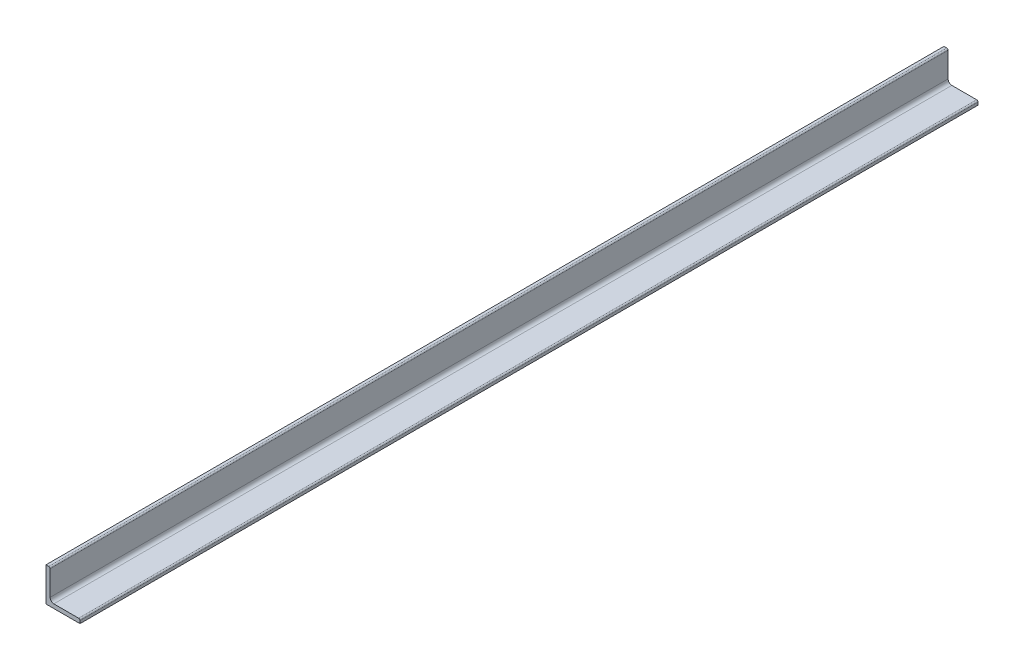
SolidWorks part; units mm, degrees
material "普通碳钢"
ref_plane "Front Plane" through (0, 0, 0) normal (0, 0, 1) x (1, 0, 0)
ref_plane "Top Plane" through (0, 0, 0) normal (0, 1, 0) x (1, 0, 0)
ref_plane "Right Plane" through (0, 0, 0) normal (1, 0, 0) x (0, 0, -1)
sketch "Sketch1" plane through (0, 0, 0) normal (0, 0, 1) x (1, 0, 0)
  line L0 (0, 50) -> (0, 0)
  line L1 (0, 0) -> (50, 0)
  line L2 (50, 0) -> (50, 4)
  line L3 (48, 6) -> (11.5, 6)
  line L4 (6, 11.5) -> (6, 48)
  line L5 (4, 50) -> (0, 50)
  arc A0 (11.5, 6) -> (6, 11.5) centre (11.5, 11.5) cw
  arc A1 (50, 4) -> (48, 6) centre (48, 4) ccw
  arc A2 (6, 48) -> (4, 50) centre (4, 48) ccw
  point P11 (50, 6)
  point P14 (6, 50)
  dimension "D5" = 5.5
  dimension "D6" = 2
  dimension "D1" = 50
  dimension "D2" = 50
  dimension "D3" = 6
  dimension "D4" = 6
extrude "Boss-Extrude1" add sketch "Sketch1" along normal mid plane 1320.8
